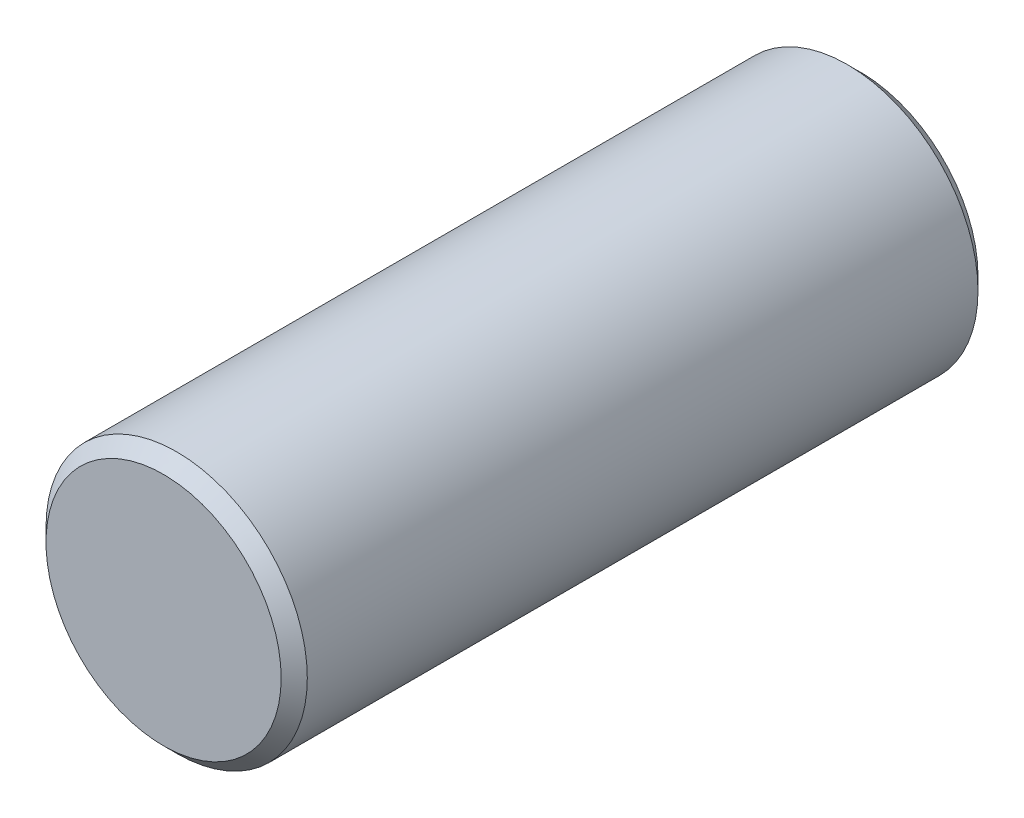
from build123d import *

# Parameters (mm, degrees)
SKETCH1_R           = 3
BOSS_EXTRUDE1_DEPTH = 8
CHAMFER1_SIZE       = 0.3


with BuildPart() as part:
    # Sketch1 → Boss-Extrude1 (new, symmetric)
    with BuildSketch(Plane.XY):
        Circle(SKETCH1_R)
    extrude(amount=BOSS_EXTRUDE1_DEPTH, both=True)

    # Chamfer1
    chamfer1_edges = [part.edges().sort_by_distance(p)[0] for p in [
        (-3, 0, -8),
        (-3, 0, 8),
    ]]
    chamfer(chamfer1_edges, length=CHAMFER1_SIZE)


solid = part.part
